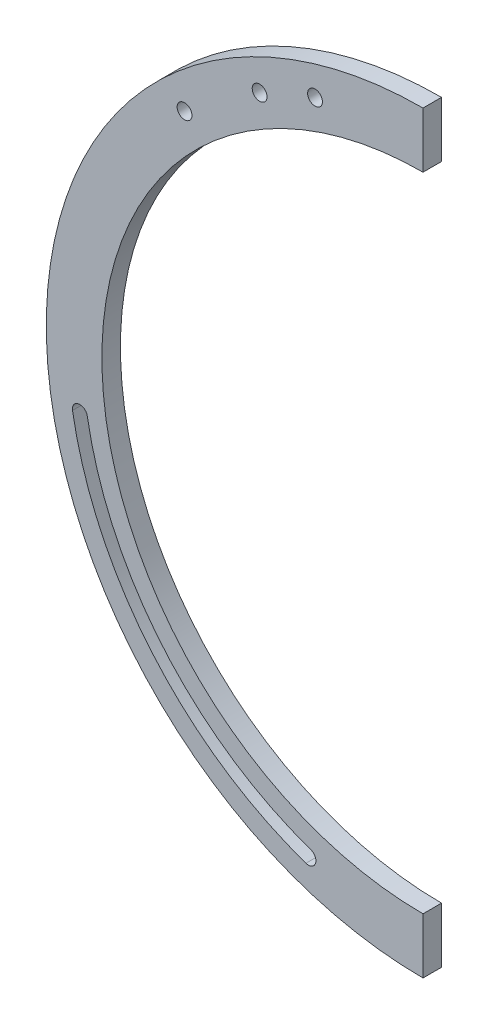
SolidWorks part; units mm, degrees
ref_plane "Front Plane" through (0, 0, 0) normal (0, 0, 1) x (1, 0, 0)
ref_plane "Top Plane" through (0, 0, 0) normal (0, 1, 0) x (1, 0, 0)
ref_plane "Right Plane" through (0, 0, 0) normal (1, 0, 0) x (0, 0, -1)
sketch "Sketch1" plane through (0, 0, 0) normal (0, 0, 1) x (1, 0, 0)
  circle A0 centre (291.5852, 182.7307) radius 203.2949
  circle A1 centre (291.5852, 182.7307) radius 173.2949
  arc A2 (93.8621, 230) -> (110.6713, 90) centre (291.5852, 182.7307) ccw construction
  dimension "D1" = 30
extrude "Boss-Extrude1" add sketch "Sketch1" against normal blind 10
sketch "Sketch2" plane through (0, 0, -10) normal (0, 0, -1) x (-1, 0, 0)
  line L0 (-291.5852, 9.4358) -> (-291.5852, -33.9055)
  line L1 (-291.5852, 356.0256) -> (-291.5852, 399.3669)
  circle A0 centre (-291.5852, 182.7307) radius 173.2949 construction
  arc A1 (-291.5852, 356.0256) -> (-291.5852, 9.4358) centre (-291.5852, 182.7307) ccw
  arc A2 (-291.5852, 399.3669) -> (-291.5852, -33.9055) centre (-291.5852, 182.7307) ccw
extrude "Cut-Extrude1" cut sketch "Sketch2" against normal blind 185
sketch "Sketch3" plane through (0, 0, -10) normal (0, 0, -1) x (-1, 0, 0)
  arc A0 (-229.7309, 5.3027) -> (-106.4155, 150.8116) centre (-291.5852, 182.7307) ccw construction
  arc A1 (-228.3982, 1.4801) -> (-102.4261, 150.1239) centre (-291.5852, 182.7307) ccw
  arc A2 (-231.0635, 9.1254) -> (-110.4049, 151.4993) centre (-291.5852, 182.7307) ccw
  arc A3 (-231.0635, 9.1254) -> (-228.3982, 1.4801) centre (-229.7309, 5.3027) ccw
  arc A4 (-102.4261, 150.1239) -> (-110.4049, 151.4993) centre (-106.4155, 150.8116) ccw
  circle A6 centre (-291.5852, 182.7307) radius 187.9006 construction
  point P5 (-148.238, 61.2473)
extrude "Cut-Extrude2" cut sketch "Sketch3" against normal blind 185
sketch "Sketch5" plane through (0, 0, 0) normal (0, 0, 1) x (1, 0, 0)
  circle A0 centre (233.3177, 361.7834) radius 4
  circle A1 centre (203.4116, 349.105) radius 4
  circle A2 centre (162.898, 320.1883) radius 4
extrude "Cut-Extrude3" cut sketch "Sketch5" against normal through all both and the other way through all
